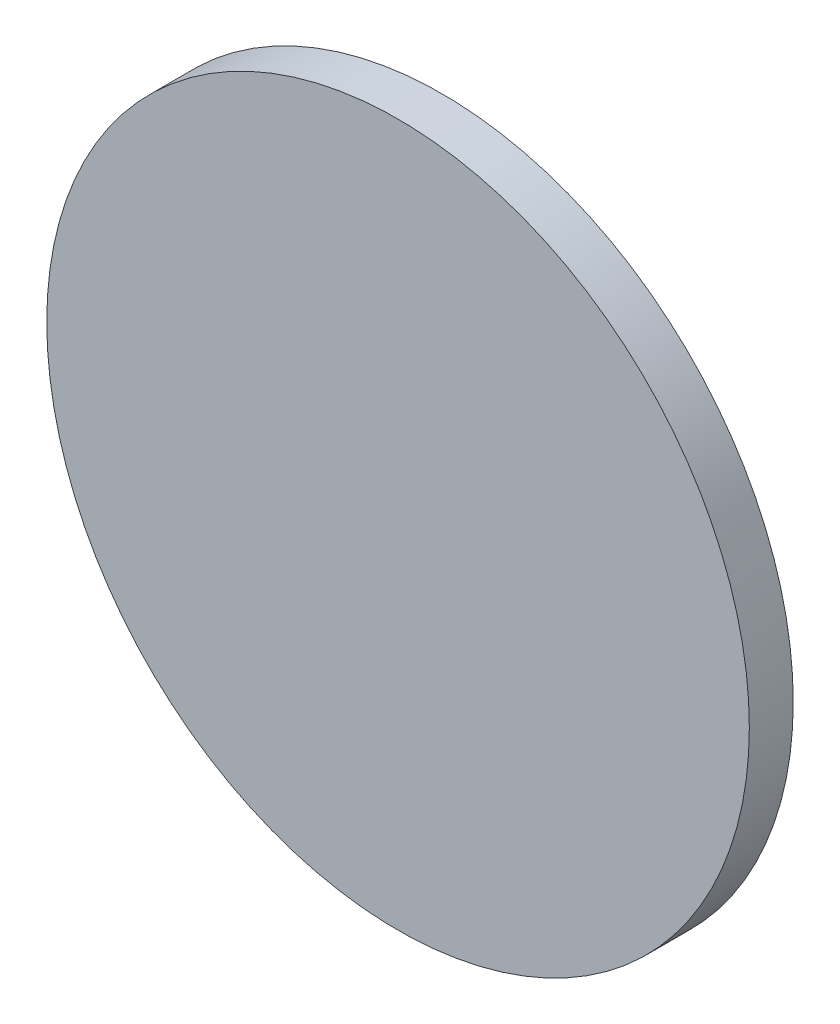
from build123d import *

# Parameters (mm, degrees)
SKETCH1_R           = 8
BOSS_EXTRUDE1_DEPTH = 1


with BuildPart() as part:
    # Sketch1 → Boss-Extrude1 (new body)
    with BuildSketch(Plane.XY):
        Circle(SKETCH1_R)
    extrude(amount=BOSS_EXTRUDE1_DEPTH)


solid = part.part
